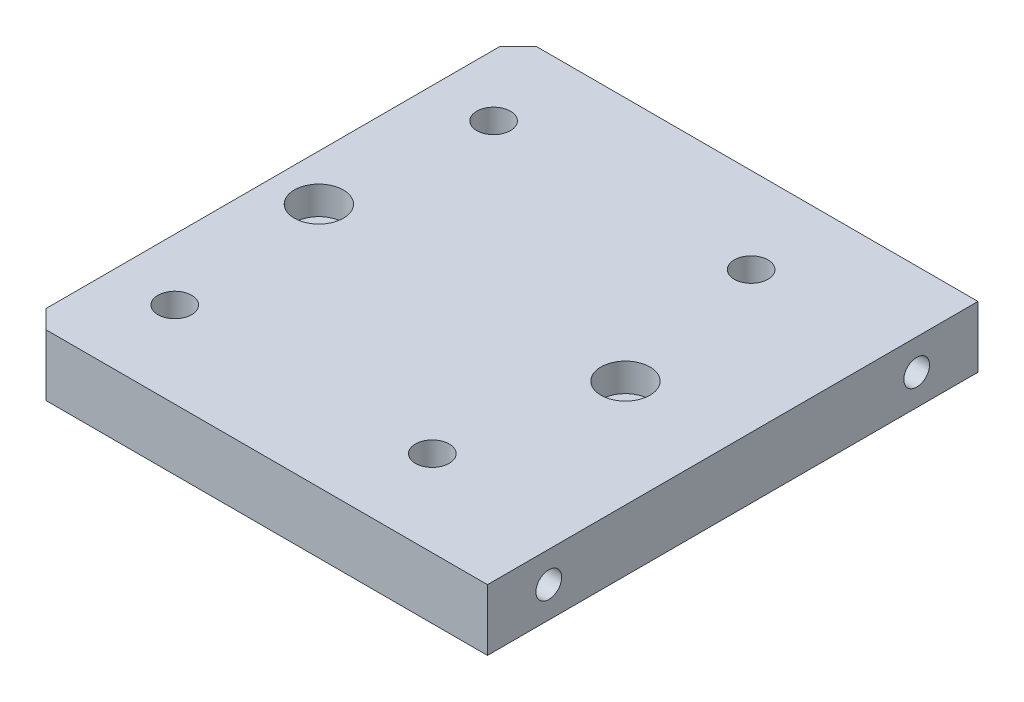
from build123d import *

# Parameters (mm, degrees)
SKETCH_1_W                = 75
SKETCH_1_H                = 80
EXTRUDE_1_DEPTH           = 5
CHAMFER_1_SIZE            = 3
HOLE_WIZARD_M5_1_D        = 4.2
HOLE_WIZARD_M5_1_DEPTH    = 12.4
HOLE_WIZARD_M5_1_TIP      = 1.2618073
HOLE_WIZARD_1_D           = 5.5
HOLE_WIZARD_1_CBORE_D     = 10
HOLE_WIZARD_1_CBORE_DEPTH = 5.7
HOLE_WIZARD_2_D           = 4.5
HOLE_WIZARD_2_CBORE_D     = 8
HOLE_WIZARD_2_CBORE_DEPTH = 4.6


with BuildPart() as part:
    # 草图1 → 凸台-拉伸1 (new, symmetric)
    with BuildSketch(Plane(origin=(0, 0, 0), x_dir=(1, 0, 0), z_dir=(0, 1, 0))):
        Rectangle(SKETCH_1_W, SKETCH_1_H)
    extrude(amount=EXTRUDE_1_DEPTH, both=True)

    # 倒角1
    chamfer_1_edges = [part.edges().sort_by_distance(p)[0] for p in [
        (-37.5, 0, 40),
        (-37.5, 0, -40),
    ]]
    chamfer(chamfer_1_edges, length=CHAMFER_1_SIZE)

    # M5 螺纹孔1
    with Locations(Plane(origin=(37.5, 0, 0), x_dir=(0, 0, -1), z_dir=(1, 0, 0))):
        with Locations((-30, 0), (30, 0)):
            Hole(HOLE_WIZARD_M5_1_D / 2, depth=HOLE_WIZARD_M5_1_DEPTH)
            with Locations((0, 0, -(HOLE_WIZARD_M5_1_DEPTH + HOLE_WIZARD_M5_1_TIP / 2))):  # 118° drill point
                Cone(0, HOLE_WIZARD_M5_1_D / 2, HOLE_WIZARD_M5_1_TIP, mode=Mode.SUBTRACT)

    # 打孔尺寸(%根据)内六角圆柱头螺钉的类型1 (through all)
    with Locations(Plane.XZ.offset(5)):
        with Locations((-27.5, -26), (14.5, -26), (14.5, 26), (-27.5, 26)):
            CounterBoreHole(HOLE_WIZARD_1_D / 2, HOLE_WIZARD_1_CBORE_D / 2, HOLE_WIZARD_1_CBORE_DEPTH)

    # 打孔尺寸(%根据)内六角圆柱头螺钉的类型2 (through all)
    with Locations(Plane(origin=(0, 5, 0), x_dir=(1, 0, 0), z_dir=(0, 1, 0))):
        with Locations((-30, 0), (20, 0)):
            CounterBoreHole(HOLE_WIZARD_2_D / 2, HOLE_WIZARD_2_CBORE_D / 2, HOLE_WIZARD_2_CBORE_DEPTH)


solid = part.part
